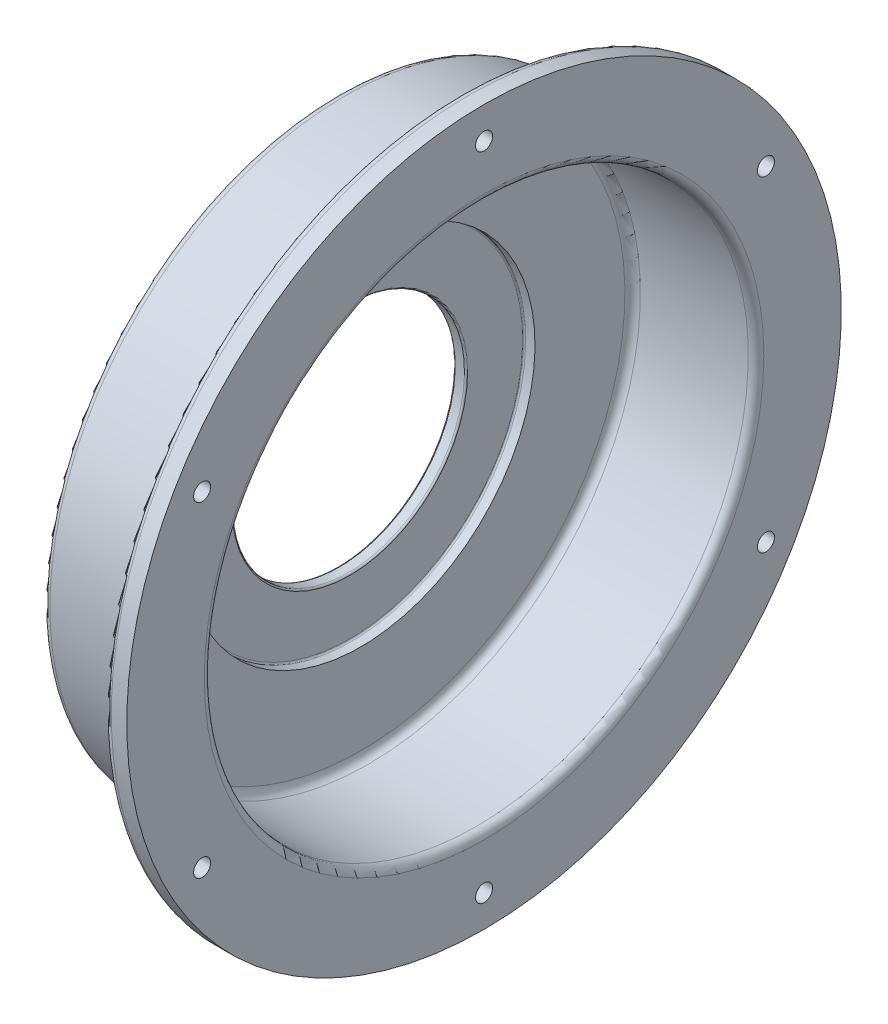
from build123d import *

# Parameters (mm, degrees)
SKETCH2_R          = 5.5
CUT_EXTRUDE1_DEPTH = 85


with BuildPart() as part:
    # Sketch1 → Revolve2 (revolve)
    with BuildSketch(Plane.XY):
        with BuildLine():
            Line((218.919928267, 112.5), (212.919928267, 112.5))
            ThreePointArc((212.919928267, 112.5), (212.212821486, 112.207106781), (211.919928267, 111.5))
            Line((211.919928267, 111.5), (211.919928267, 76))
            ThreePointArc((211.919928267, 76), (211.627035048, 75.292893219), (210.919928267, 75))
            Line((210.919928267, 75), (204.919928267, 75))
            ThreePointArc((204.919928267, 75), (204.212821486, 75.292893219), (203.919928267, 76))
            Line((203.919928267, 76), (203.919928267, 131))
            Line((203.919928267, 131), (203.919928267, 185.5))
            ThreePointArc((203.919928267, 185.5), (205.384394361, 189.035533906), (208.919928267, 190.5))
            Line((208.919928267, 190.5), (278.519928267, 190.5))
            ThreePointArc((278.519928267, 190.5), (282.055462173, 191.964466094), (283.519928267, 195.5))
            Line((283.519928267, 195.5), (283.519928267, 225.5))
            ThreePointArc((283.519928267, 225.5), (284.984394361, 229.035533906), (288.519928267, 230.5))
            Line((288.519928267, 230.5), (298.519928267, 230.5))
            Line((298.519928267, 230.5), (298.519928267, 205))
            Line((298.519928267, 205), (298.519928267, 180.5))
            ThreePointArc((298.519928267, 180.5), (297.055462173, 176.964466094), (293.519928267, 175.5))
            Line((293.519928267, 175.5), (223.919928267, 175.5))
            ThreePointArc((223.919928267, 175.5), (220.384394361, 174.035533906), (218.919928267, 170.5))
            Line((218.919928267, 170.5), (218.919928267, 131))
            Line((218.919928267, 131), (218.919928267, 112.5))
        make_face()
    revolve(axis=Axis((373.519928267, 0, 0), (-1, 0, 0)))

    # Sketch2 → Cut-Extrude1 (cut)
    with BuildSketch(Plane.ZY.offset(-283.519928267)):
        with Locations(Location((0, 210, 0), (0, 0, 270))):
            Circle(SKETCH2_R)
        with Locations(Location((181.865334795, 105, 0), (0, 0, 270))):
            Circle(SKETCH2_R)
        with Locations(Location((181.865334795, -105, 0), (0, 0, 270))):
            Circle(SKETCH2_R)
        with Locations(Location((0, -210, 0), (0, 0, 270))):
            Circle(SKETCH2_R)
        with Locations(Location((-181.865334795, -105, 0), (0, 0, 270))):
            Circle(SKETCH2_R)
        with Locations(Location((-181.865334795, 105, 0), (0, 0, 270))):
            Circle(SKETCH2_R)
    extrude(amount=-CUT_EXTRUDE1_DEPTH, mode=Mode.SUBTRACT)


solid = part.part
